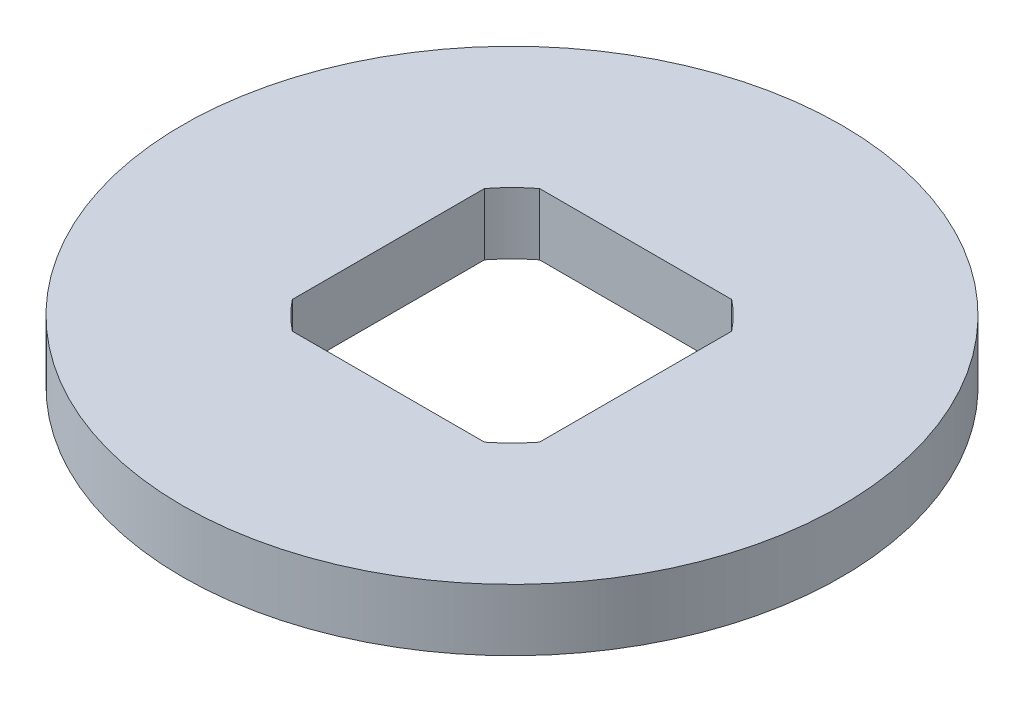
from build123d import *

# Parameters (mm, degrees)
SKETCH1_R           = 8
BOSS_EXTRUDE1_DEPTH = 1.5


with BuildPart() as part:
    # Sketch1 → Boss-Extrude1 (new body)
    with BuildSketch(Plane.XZ.offset(1.5)):
        with Locations(Location((0, 0, 0), (0, 0, 90))):
            Circle(SKETCH1_R)
        with BuildLine():
            Line((3, 2.332380758), (3, -2.332380758))
            ThreePointArc((3, -2.332380758), (2.687005769, -2.687005769), (2.332380758, -3))
            Line((2.332380758, -3), (-2.332380758, -3))
            ThreePointArc((-2.332380758, -3), (-2.687005769, -2.687005769), (-3, -2.332380758))
            Line((-3, -2.332380758), (-3, 2.332380758))
            ThreePointArc((-3, 2.332380758), (-2.687005769, 2.687005769), (-2.332380758, 3))
            Line((-2.332380758, 3), (2.332380758, 3))
            ThreePointArc((2.332380758, 3), (2.687005769, 2.687005769), (3, 2.332380758))
        make_face(mode=Mode.SUBTRACT)
    extrude(amount=-BOSS_EXTRUDE1_DEPTH)


solid = part.part
